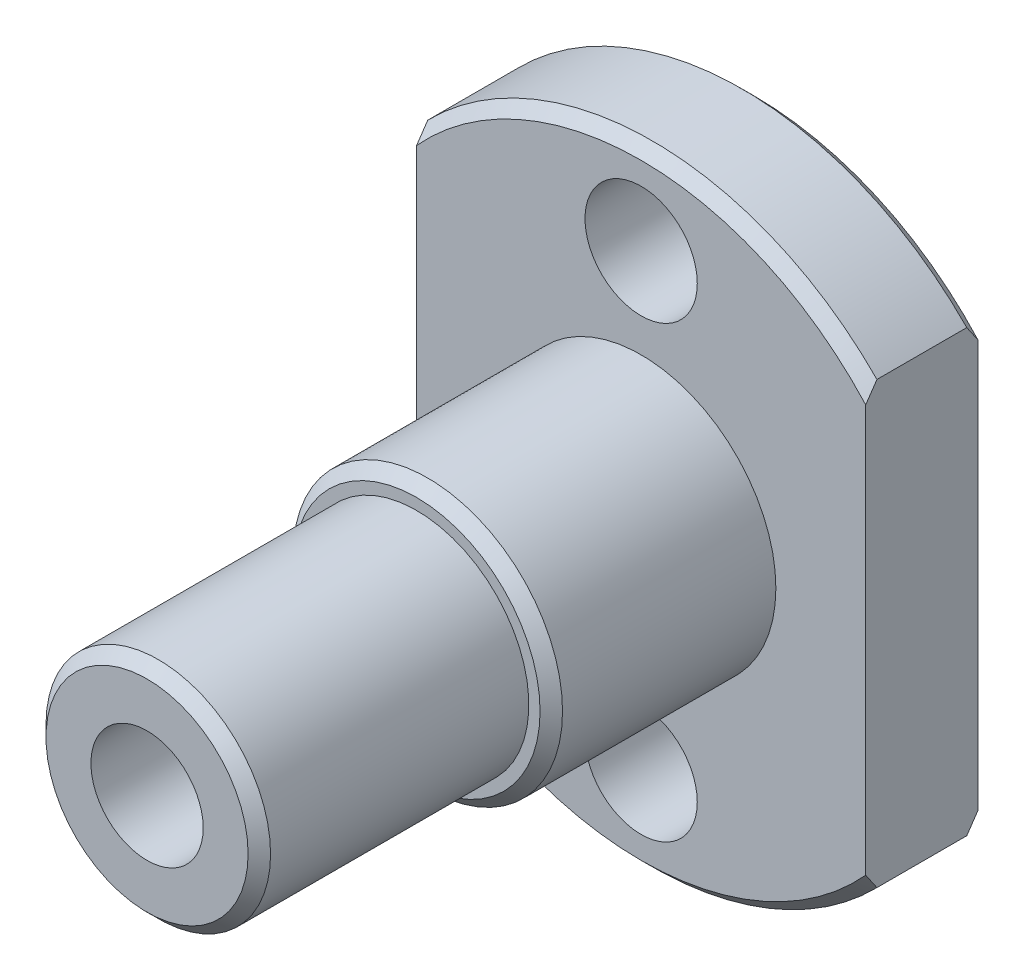
from build123d import *

# Parameters (mm, degrees)
SKETCH_1_R                = 5
EXTRUDE_1_DEPTH           = 22
SKETCH_2_R                = 6
EXTRUDE_2_DEPTH           = 10
SKETCH_3_R                = 14
EXTRUDE_3_DEPTH           = 5
SKETCH_4_OUTSIDE_W        = 39.586
SKETCH_4_OUTSIDE_H        = 39.586
SKETCH_4_OUTSIDE_W_2      = 20
SKETCH_4_OUTSIDE_H_2      = 37.741501618
CUT_EXTRUDE_1_DEPTH       = 5
HOLE_WIZARD_5_0_5_1_D     = 5
HOLE_WIZARD_5_0_5_1_DEPTH = 20
HOLE_WIZARD_5_0_5_1_TIP   = 1.502151548
HOLE_WIZARD_M6_1_D        = 5
HOLE_WIZARD_M6_1_DEPTH    = 15
HOLE_WIZARD_M6_1_TIP      = 1.502151548
CHAMFER_1_SIZE            = 0.5
CHAMFER_2_SIZE            = 0.5


with BuildPart() as part:
    # 草图1 → 凸台-拉伸1 (new body)
    with BuildSketch(Plane.XY):
        Circle(SKETCH_1_R)
    extrude(amount=EXTRUDE_1_DEPTH)

    # 草图2 → 凸台-拉伸2 (add)
    with BuildSketch(Plane(origin=(0, 0, 0), x_dir=(-1, 0, 0), z_dir=(0, 0, -1))):
        Circle(SKETCH_2_R)
    extrude(amount=-EXTRUDE_2_DEPTH)

    # 草图3 → 凸台-拉伸3 (add)
    with BuildSketch(Plane(origin=(0, 0, 0), x_dir=(-1, 0, 0), z_dir=(0, 0, -1))):
        Circle(SKETCH_3_R)
    extrude(amount=EXTRUDE_3_DEPTH)

    # 草图4 outside → 切除-拉伸1 (cut)
    with BuildSketch(Plane(origin=(0, 0, -5), x_dir=(-1, 0, 0), z_dir=(0, 0, -1))):
        Rectangle(SKETCH_4_OUTSIDE_W, SKETCH_4_OUTSIDE_H)
        with Locations((0, -0.226902815)):
            Rectangle(SKETCH_4_OUTSIDE_W_2, SKETCH_4_OUTSIDE_H_2, mode=Mode.SUBTRACT)
    extrude(amount=-CUT_EXTRUDE_1_DEPTH, mode=Mode.SUBTRACT)

    # Ø5.0 (5) 直径孔1
    with Locations(Plane.XY):
        with Locations((0, 10), (0, -10)):
            Hole(HOLE_WIZARD_5_0_5_1_D / 2, depth=HOLE_WIZARD_5_0_5_1_DEPTH)
            with Locations((0, 0, -(HOLE_WIZARD_5_0_5_1_DEPTH + HOLE_WIZARD_5_0_5_1_TIP / 2))):  # 118° drill point
                Cone(0, HOLE_WIZARD_5_0_5_1_D / 2, HOLE_WIZARD_5_0_5_1_TIP, mode=Mode.SUBTRACT)

    # M6 螺纹孔1
    with Locations(Plane.XY.offset(22)):
        with Locations((0, 0)):
            Hole(HOLE_WIZARD_M6_1_D / 2, depth=HOLE_WIZARD_M6_1_DEPTH)
            with Locations((0, 0, -(HOLE_WIZARD_M6_1_DEPTH + HOLE_WIZARD_M6_1_TIP / 2))):  # 118° drill point
                Cone(0, HOLE_WIZARD_M6_1_D / 2, HOLE_WIZARD_M6_1_TIP, mode=Mode.SUBTRACT)

    # 倒角1
    chamfer_1_edges = [part.edges().sort_by_distance(p)[0] for p in [
        (-5, 0, 22),
        (6, 0, 10),
    ]]
    chamfer(chamfer_1_edges, length=CHAMFER_1_SIZE)

    # 倒角2
    chamfer_2_edges = [part.edges().sort_by_distance(p)[0] for p in [
        (0, 14, 0),
        (0, 14, -5),
        (0, -14, 0),
        (0, -14, -5),
    ]]
    chamfer(chamfer_2_edges, length=CHAMFER_2_SIZE)


solid = part.part
